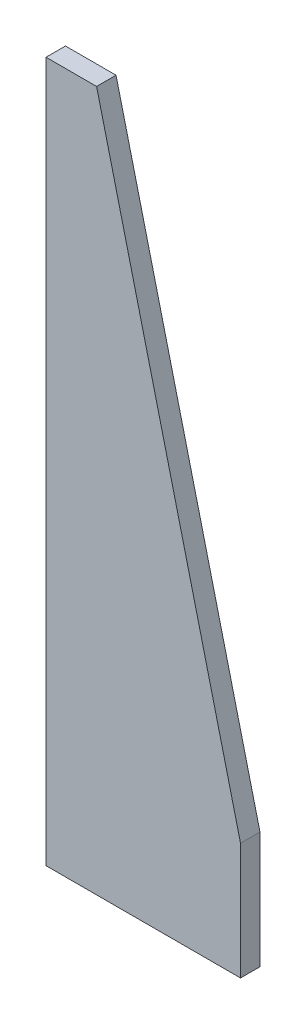
from build123d import *

# Parameters (mm, degrees)
BOSS_EXTRUDE1_DEPTH = 10


with BuildPart() as part:
    # Sketch1 → Boss-Extrude1 (new body)
    with BuildSketch(Plane.XY):
        Polygon((0, 0), (100, 0), (100, 60), (26, 360), (0, 360), align=None)
    extrude(amount=BOSS_EXTRUDE1_DEPTH)


solid = part.part
